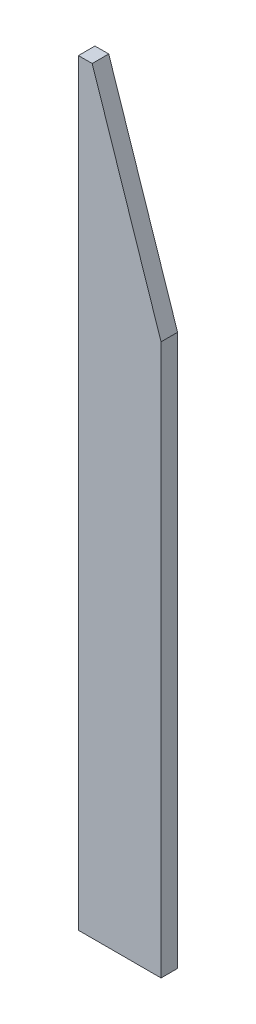
SolidWorks part; units mm, degrees
material "1023 碳钢板 (SS)"
ref_plane "前视基准面" through (0, 0, 0) normal (0, 0, 1) x (1, 0, 0)
ref_plane "上视基准面" through (0, 0, 0) normal (0, 1, 0) x (1, 0, 0)
ref_plane "右视基准面" through (0, 0, 0) normal (1, 0, 0) x (0, 0, -1)
sketch "草图1" plane through (0, 0, 0) normal (0, 0, 1) x (1, 0, 0)
  line L1 (30, 275) -> (-30, 275)
  line L2 (30, 275) -> (30, -275)
  line L3 (30, -275) -> (-30, -275)
  line L4 (-30, 275) -> (-30, -275)
  line L5 (30, 275) -> (-30, -275) construction
  line L6 (30, -275) -> (-30, 275) construction
  point P0 (0, 0)
  dimension "D1" = 60
  dimension "D2" = 550
extrude "凸台-拉伸1" add sketch "草图1" along normal blind 12
sketch "草图2" plane through (0, 0, 12) normal (0, 0, 1) x (1, 0, 0)
  line L0 (-20, 275) -> (30, 125)
  line L1 (30, 275) -> (-30, 275) construction
  line L2 (30, -275) -> (30, 275) construction
  line L3 (30, 125) -> (30, 275)
  line L4 (30, 275) -> (-20, 275)
  dimension "D1" = 10
  dimension "D2" = 150
extrude "切除-拉伸1" cut sketch "草图2" against normal blind 12
